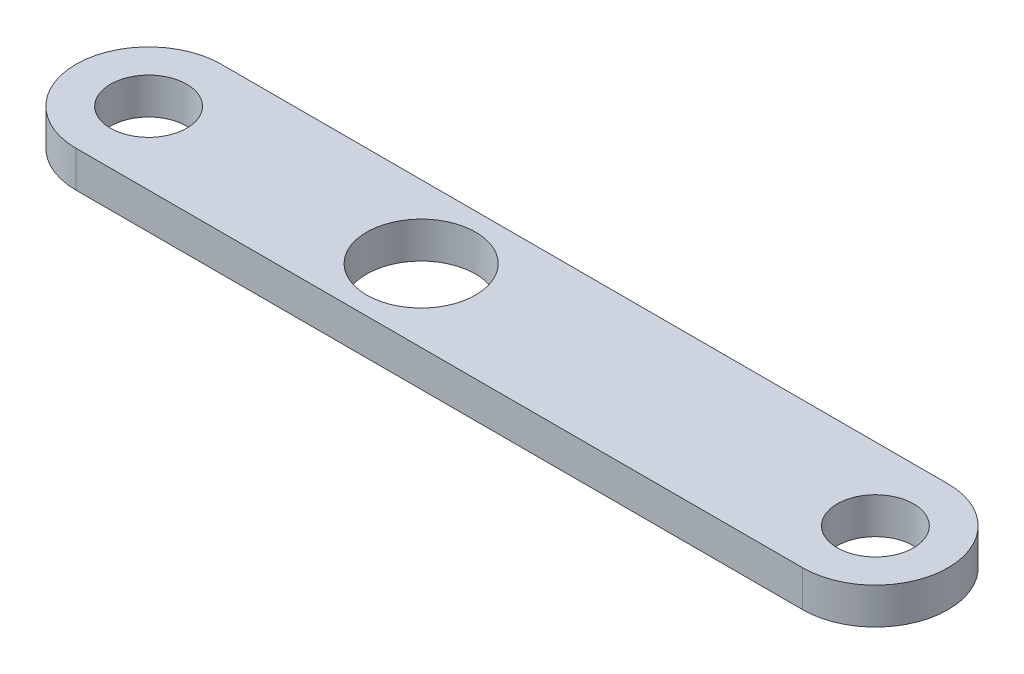
from build123d import *

# Parameters (mm, degrees)
SKETCH1_R           = 2.667
SKETCH1_R_2         = 3.81
BOSS_EXTRUDE1_DEPTH = 2.54
SCALE1_SCALE        = 2


with BuildPart() as part:
    # Sketch1 → Boss-Extrude1 (new body)
    with BuildSketch(Plane(origin=(0, 0, 0), x_dir=(1, 0, 0), z_dir=(0, 1, 0))):
        with BuildLine():
            Line((-25.4, 5.08), (25.4, 5.08))
            ThreePointArc((25.4, 5.08), (30.48, 0), (25.4, -5.08))
            Line((25.4, -5.08), (-25.4, -5.08))
            ThreePointArc((-25.4, -5.08), (-30.48, 0), (-25.4, 5.08))
        make_face()
        with Locations(Location((-25.4, 0, 0), (0, 0, 270))):
            Circle(SKETCH1_R, mode=Mode.SUBTRACT)
        with Locations(Location((25.4, 0, 0), (0, 0, 270))):
            Circle(SKETCH1_R, mode=Mode.SUBTRACT)
        with Locations(Location((-6.35, 0, 0), (0, 0, 270))):
            Circle(SKETCH1_R_2, mode=Mode.SUBTRACT)
    extrude(amount=BOSS_EXTRUDE1_DEPTH)


with BuildPart() as part_1:
    # Scale1: scaled about (0, 0, 0)
    add(part.part.scale(SCALE1_SCALE))


solid = part_1.part
